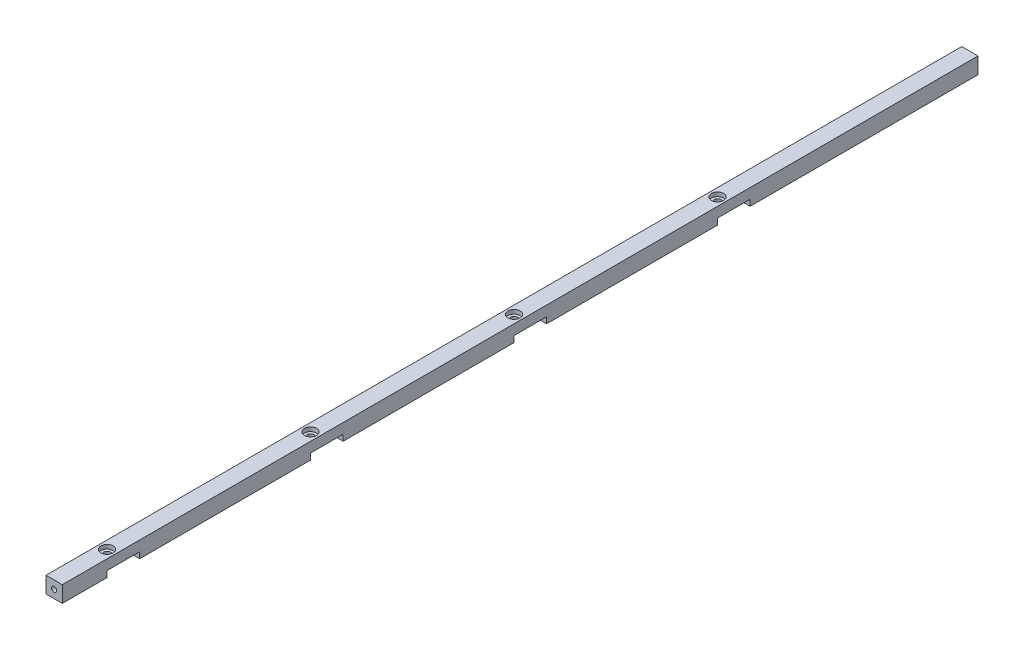
SolidWorks part; units mm, degrees
ref_plane "前视基准面" through (0, 0, 0) normal (0, 0, 1) x (1, 0, 0)
ref_plane "上视基准面" through (0, 0, 0) normal (0, 1, 0) x (1, 0, 0)
ref_plane "右视基准面" through (0, 0, 0) normal (1, 0, 0) x (0, 0, -1)
sketch "草图1" plane through (0, 0, 0) normal (0, 0, 1) x (1, 0, 0)
  line L1 (-4, 4) -> (4, 4)
  line L2 (-4, 4) -> (-4, -4)
  line L3 (-4, -4) -> (4, -4)
  line L4 (4, 4) -> (4, -4)
  line L5 (-4, 4) -> (4, -4) construction
  line L6 (-4, -4) -> (4, 4) construction
  point P0 (0, 0)
  dimension "D1" = 8
  dimension "D2" = 8
extrude "凸台-拉伸1" add sketch "草图1" along normal blind 450
sketch "草图3" plane through (0, -4, 0) normal (0, -1, 0) x (1, 0, 0)
  line L0 (-4, 450) -> (-4, 0) construction
  line L1 (-4, 428) -> (4, 428)
  line L2 (-4, 428) -> (-4, 412)
  line L3 (-4, 412) -> (4, 412)
  line L4 (4, 428) -> (4, 412)
  line L5 (4, 450) -> (4, 0) construction
  line L6 (-4, 450) -> (4, 450) construction
  dimension "D1" = 16
  dimension "D2" = 22
extrude "切除-拉伸2" cut sketch "草图3" against normal blind 3
hole_wizard "M3 螺纹孔1" positions "草图7" profile "草图6" tap size "M3" standard "Iso"
sketch "草图7" plane through (0, 0, 0) normal (0, 0, -1) x (-1, 0, 0)
  point P0 (0, 0)
sketch "草图6" plane through (0, 0, 0) normal (1, 0, 0) x (0, 1, 0)
  line L0 (0, 0) -> (0, 12.7511)
  line L1 (0, 12.7511) -> (1.25, 12)
  line L2 (1.25, 12) -> (1.25, 0)
  line L5 (1.25, 0) -> (0, 0)
  line L10 (0, 12.7511) -> (-1.25, 12) construction
  line L11 (0, -6.35) -> (0, 107.95) construction
  dimension "螺纹孔钻头直径" = 2.5
  dimension "螺纹孔钻头深度" = 12
  dimension "导头角度" = 118
cosmetic thread "孔螺蚊线1" parameters "D1"=8, "D2"=3
hole_wizard "M3 螺纹孔2" positions "草图9" profile "草图8" tap size "M3" standard "Iso"
sketch "草图9" plane through (0, 0, 450) normal (0, 0, 1) x (1, 0, 0)
  point P0 (0, 0)
sketch "草图8" plane through (0, 0, 450) normal (1, 0, 0) x (0, -1, 0)
  line L0 (0, 0) -> (0, 12.7511)
  line L1 (0, 12.7511) -> (1.25, 12)
  line L2 (1.25, 12) -> (1.25, 0)
  line L5 (1.25, 0) -> (0, 0)
  line L10 (0, 12.7511) -> (-1.25, 12) construction
  line L11 (0, -6.35) -> (0, 107.95) construction
  dimension "螺纹孔钻头直径" = 2.5
  dimension "螺纹孔钻头深度" = 12
  dimension "导头角度" = 118
cosmetic thread "孔螺蚊线2" parameters "D1"=8, "D2"=3
sketch "草图10" plane through (4, 0, 0) normal (1, 0, 0) x (0, 0, -1)
  line L0 (-412, -4) -> (0, -4) construction
  line L1 (-312, -4) -> (-328, -4)
  line L2 (-312, -4) -> (-312, -1)
  line L3 (-312, -1) -> (-328, -1)
  line L4 (-328, -4) -> (-328, -1)
  line L7 (-428, -1) -> (-428, -4) construction
  line L9 (-228, -4) -> (-212, -4)
  line L10 (-228, -4) -> (-228, -1)
  line L11 (-228, -1) -> (-212, -1)
  line L12 (-212, -4) -> (-212, -1)
  line L13 (-128, -4) -> (-112, -4)
  line L14 (-128, -4) -> (-128, -1)
  line L15 (-128, -1) -> (-112, -1)
  line L16 (-112, -4) -> (-112, -1)
  dimension "D1" = 100
  dimension "D2" = 16
  dimension "D3" = 3
  dimension "D4" = 100
  dimension "D5" = 16
  dimension "D6" = 3
  dimension "D7" = 100
  dimension "D8" = 16
  dimension "D9" = 3
extrude "切除-拉伸3" cut sketch "草图10" against normal through all
hole_wizard "打孔尺寸根据内六角圆柱头螺钉的类型1" positions "草图12" profile "草图11" counterbore size "M3" standard "Gb" end condition through all
sketch "草图12" plane through (0, 4, 0) normal (0, 1, 0) x (1, 0, 0)
  point P0 (0, -124)
  point P3 (0, -224)
  point P6 (0, -324)
  point P9 (0, -424)
sketch "草图11" plane through (0, 4, 124) normal (1, 0, 0) x (0, 0, 1)
  line L0 (0, 0) -> (0, 8)
  line L1 (0, 8) -> (1.7, 8)
  line L3 (1.7, 8) -> (1.7, 2)
  line L4 (1.7, 2) -> (3, 2)
  line L5 (3, 2) -> (3, 0)
  line L7 (3, 0) -> (0, 0)
  line L11 (0, -6.35) -> (0, 107.95) construction
  dimension "通孔孔直径" = 3.4
  dimension "通孔孔深度" = 8
  dimension "柱形沉头孔直径" = 6
  dimension "柱形沉头孔深度" = 2
